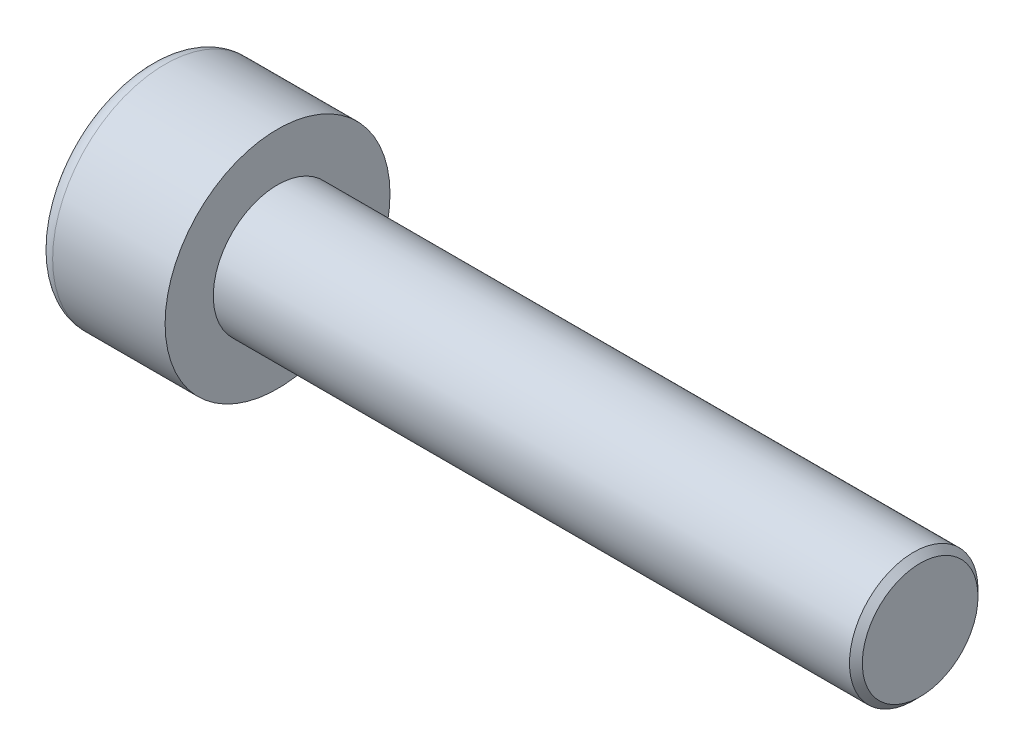
from build123d import *

# Parameters (mm, degrees)
SKETCH1_R           = 3.5
BASEHEAD_DEPTH      = 4
SKETCH2_R           = 2
BASEBODY_DEPTH      = 20
HEXAGONSOCKET_DEPTH = 2
TOPFILLET_R         = 0.5
CHAMFER1_SIZE       = 0.2


with BuildPart() as part:
    # Sketch1 → BaseHead (new body)
    with BuildSketch(Plane(origin=(0, 0, 0), x_dir=(0, 0, -1), z_dir=(1, 0, 0))):
        Circle(SKETCH1_R)
    extrude(amount=BASEHEAD_DEPTH)

    # Sketch2 → BaseBody (add)
    with BuildSketch(Plane(origin=(4, 0, 0), x_dir=(0, 0, -1), z_dir=(1, 0, 0))):
        Circle(SKETCH2_R)
    extrude(amount=BASEBODY_DEPTH)

    # Sketch3 → HexagonSocket (cut)
    with BuildSketch(Plane(origin=(0, 0, 0), x_dir=(0, 0, -1), z_dir=(1, 0, 0))):
        Polygon((1.732050808, 0), (0.866025404, 1.5), (-0.866025404, 1.5), (-1.732050808, 0), (-0.866025404, -1.5), (0.866025404, -1.5), align=None)
    extrude(amount=HEXAGONSOCKET_DEPTH, mode=Mode.SUBTRACT)

    # Sketch4 → Cut-Revolve1 (revolve, cut)
    with BuildSketch(Plane(origin=(-4.19613823, 0.75, 0), x_dir=(-1, 0, 0), z_dir=(0, 0, 1)), mode=Mode.PRIVATE) as cut_revolve1_sk:
        Polygon((-6.19613823, 2.25), (-7.062163633, 0.75), (-6.19613823, 0.75), align=None)
    revolve(cut_revolve1_sk.sketch.rotate(Axis((0.838992387, 0, 0), (-1, 0, 0)), 90), axis=Axis((0.838992387, 0, 0), (-1, 0, 0)), mode=Mode.SUBTRACT)

    # TopFillet
    topfillet_edges = [part.edges().sort_by_distance(p)[0] for p in [
        (0, 0, 3.5),
    ]]
    fillet(topfillet_edges, radius=TOPFILLET_R)

    # Chamfer1
    chamfer1_edges = [part.edges().sort_by_distance(p)[0] for p in [
        (24, 0, 2),
    ]]
    chamfer(chamfer1_edges, length=CHAMFER1_SIZE)


solid = part.part
